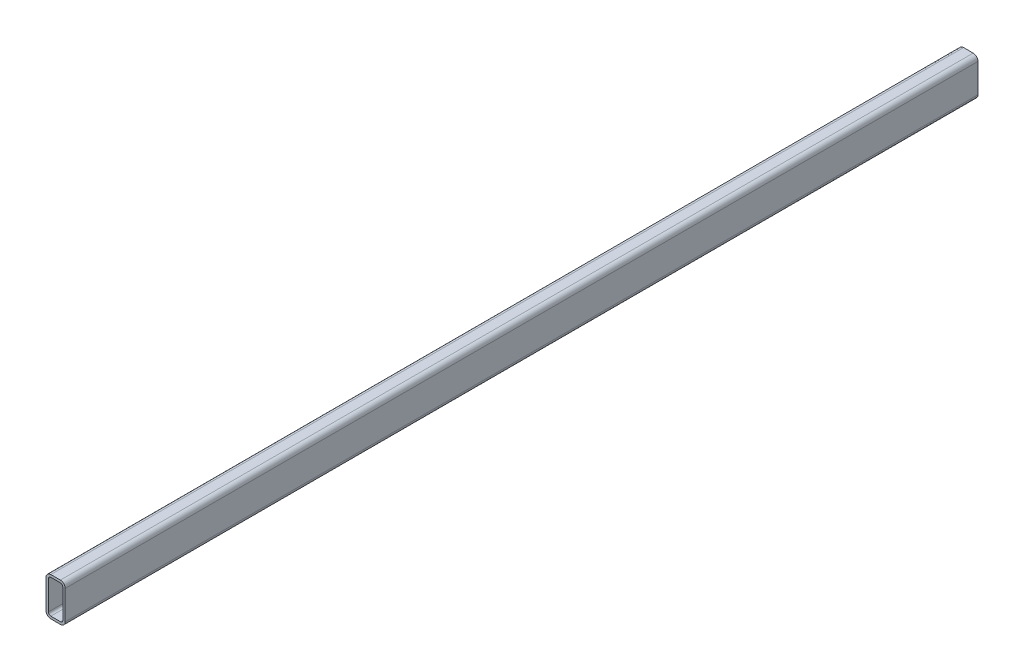
SolidWorks part; units mm, degrees
material "Q235B"
ref_plane "Plane1" through (0, 0, 0) normal (0, 0, 1) x (1, 0, 0)
ref_plane "Plane2" through (0, 0, 0) normal (0, 1, 0) x (1, 0, 0)
ref_plane "Plane3" through (0, 0, 0) normal (1, 0, 0) x (0, 0, -1)
sketch "Sketch1" plane through (0, 0, 0) normal (0, 0, 1) x (1, 0, 0)
  line L0 (-10, -35) -> (10, -35)
  line L1 (-15, -30) -> (-15, 30)
  line L2 (10, 35) -> (-10, 35)
  line L3 (15, 30) -> (15, -30)
  line L4 (-10, -40) -> (10, -40)
  line L5 (-20, -30) -> (-20, 30)
  line L6 (10, 40) -> (-10, 40)
  line L7 (20, 30) -> (20, -30)
  arc A0 (20, 30) -> (10, 40) centre (10, 30) ccw
  arc A1 (10, -40) -> (20, -30) centre (10, -30) ccw
  arc A2 (-20, -30) -> (-10, -40) centre (-10, -30) ccw
  arc A3 (-10, 40) -> (-20, 30) centre (-10, 30) ccw
  arc A4 (-10, 35) -> (-15, 30) centre (-10, 30) ccw
  arc A5 (15, 30) -> (10, 35) centre (10, 30) ccw
  arc A6 (10, -35) -> (15, -30) centre (10, -30) ccw
  arc A7 (-15, -30) -> (-10, -35) centre (-10, -30) ccw
  point P0 (0, 40)
  point P1 (20, 0)
  point P2 (0, -40)
  point P3 (-20, 0)
  point P4 (-20, 40)
  point P5 (20, 40)
  point P6 (20, -40)
  point P7 (-20, -40)
  point P8 (0, 0)
extrude "Boss-Extrude1" add sketch "Sketch1" along normal blind 1900 contours L5 A3 L6 A0 L7 A1 L4 A2 | L1 A4 L2 A5 L3 A6 L0 A7
